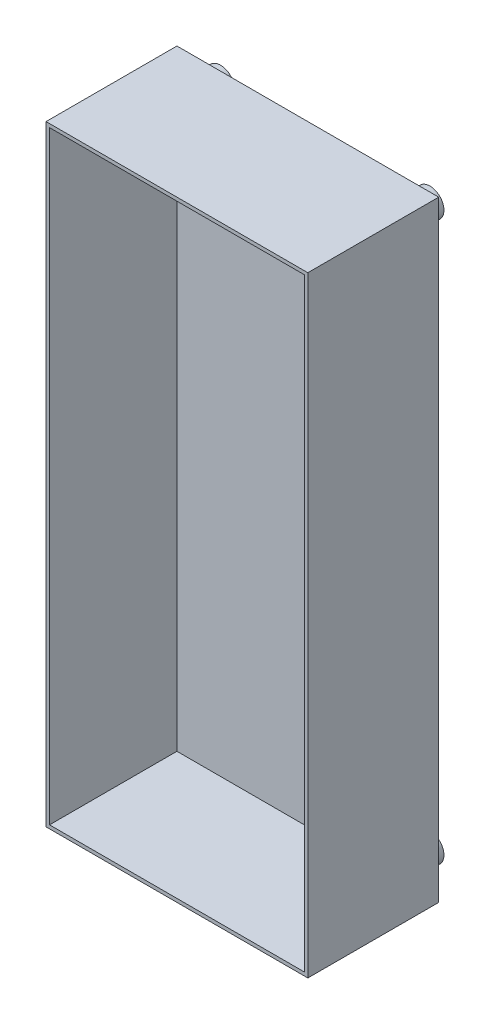
from build123d import *

# Parameters (mm, degrees)
SKETCH1_W           = 150
SKETCH1_H           = 350
BOSS_EXTRUDE1_DEPTH = 75
SHELL1_T            = -2
SKETCH2_R           = 8
BOSS_EXTRUDE2_DEPTH = 10


with BuildPart() as part:
    # Sketch1 → Boss-Extrude1 (new body)
    with BuildSketch(Plane.XY):
        Rectangle(SKETCH1_W, SKETCH1_H)
    extrude(amount=BOSS_EXTRUDE1_DEPTH)

    # Shell1
    shell1_openings = [part.faces().sort_by_distance(p)[0] for p in [
        (0, 0, 75),
    ]]
    offset(amount=SHELL1_T, openings=shell1_openings, kind=Kind.INTERSECTION)

    # Sketch2 → Boss-Extrude2 (add)
    # profile 1 of 4: a face of its own
    with BuildSketch(Plane(origin=(0, 0, 0), x_dir=(-1, 0, 0), z_dir=(0, 0, -1))):
        with Locations((-60, 160)):
            Circle(SKETCH2_R)
        Polygon((-62.973353886, 154.85), (-57.026646114, 154.85), (-54.053292227, 160), (-57.026646114, 165.15), (-62.973353886, 165.15), (-65.946707773, 160), align=None, mode=Mode.SUBTRACT)
    # profile 2 of 4: a face of its own
    with BuildSketch(Plane(origin=(0, 0, 0), x_dir=(-1, 0, 0), z_dir=(0, 0, -1))):
        with Locations(Location((-60, -160, 0), (0, 0, 180))):
            Circle(SKETCH2_R)
        Polygon((-65.946707773, -160), (-62.973353886, -154.85), (-57.026646114, -154.85), (-54.053292227, -160), (-57.026646114, -165.15), (-62.973353886, -165.15), align=None, mode=Mode.SUBTRACT)
    # profile 3 of 4: a face of its own
    with BuildSketch(Plane(origin=(0, 0, 0), x_dir=(-1, 0, 0), z_dir=(0, 0, -1))):
        with Locations((60, -160)):
            Circle(SKETCH2_R)
        Polygon((62.973353886, -165.15), (65.946707773, -160), (62.973353886, -154.85), (57.026646114, -154.85), (54.053292227, -160), (57.026646114, -165.15), align=None, mode=Mode.SUBTRACT)
    # profile 4 of 4: a face of its own
    with BuildSketch(Plane(origin=(0, 0, 0), x_dir=(-1, 0, 0), z_dir=(0, 0, -1))):
        with Locations(Location((60, 160, 0), (0, 0, 180))):
            Circle(SKETCH2_R)
        Polygon((65.946707773, 160), (62.973353886, 154.85), (57.026646114, 154.85), (54.053292227, 160), (57.026646114, 165.15), (62.973353886, 165.15), align=None, mode=Mode.SUBTRACT)
    extrude(amount=BOSS_EXTRUDE2_DEPTH)


solid = part.part
